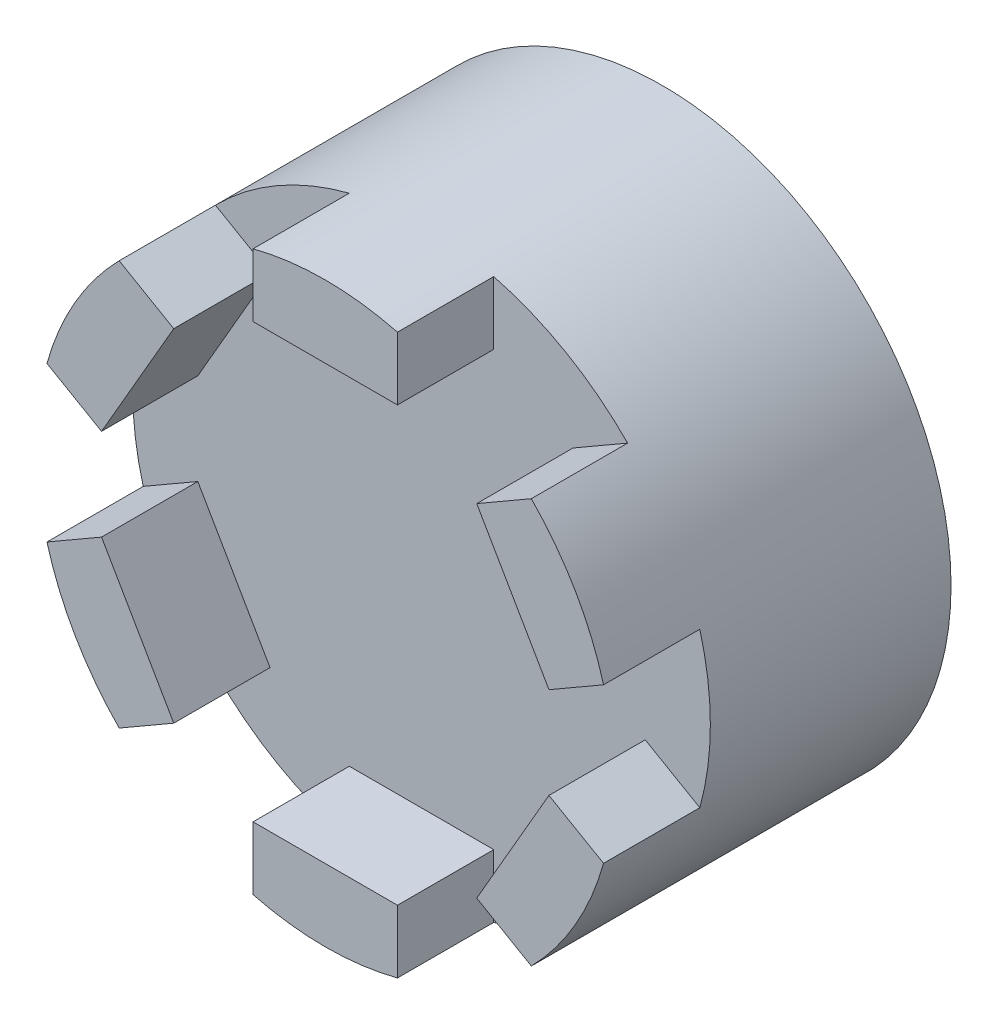
SolidWorks part; units mm, degrees
ref_plane "前视基准面" through (0, 0, 0) normal (0, 0, 1) x (1, 0, 0)
ref_plane "上视基准面" through (0, 0, 0) normal (0, 1, 0) x (1, 0, 0)
ref_plane "右视基准面" through (0, 0, 0) normal (1, 0, 0) x (0, 0, -1)
other "Configuration Table"
sketch "草图1" plane through (0, 0, 0) normal (0, 0, 1) x (1, 0, 0)
  circle A0 centre (0, 0) radius 15
  dimension "D1" = 30
sketch "草图2" plane through (0, 0, 0) normal (0, 0, 1) x (1, 0, 0)
  circle A0 centre (0, 0) radius 60
  dimension "D1" = 120
extrude "凸台-拉伸1" add sketch "草图2" along normal blind 50 contours A0
extrude "切除-拉伸1" cut sketch "草图1" along normal blind 30 contours A0
sketch "草图3" plane through (0, 0, 50) normal (0, 0, 1) x (1, 0, 0)
  line L0 (42.8115, 42.0378) -> (31.4711, 35.4904)
  line L2 (-15, 58.0948) -> (-15, 45)
  line L3 (-15, 45) -> (15, 45)
  line L4 (15, 58.0948) -> (15, 45)
  line L5 (57.8115, 16.057) -> (46.4711, 9.5096)
  line L6 (31.4711, 35.4904) -> (46.4711, 9.5096)
  line L7 (57.8115, -16.057) -> (46.4711, -9.5096)
  line L8 (42.8115, -42.0378) -> (31.4711, -35.4904)
  line L9 (46.4711, -9.5096) -> (31.4711, -35.4904)
  line L10 (15, -58.0948) -> (15, -45)
  line L11 (-15, -58.0948) -> (-15, -45)
  line L12 (15, -45) -> (-15, -45)
  line L13 (-42.8115, -42.0378) -> (-31.4711, -35.4904)
  line L14 (-57.8115, -16.057) -> (-46.4711, -9.5096)
  line L15 (-31.4711, -35.4904) -> (-46.4711, -9.5096)
  line L16 (-57.8115, 16.057) -> (-46.4711, 9.5096)
  line L17 (-42.8115, 42.0378) -> (-31.4711, 35.4904)
  line L18 (-46.4711, 9.5096) -> (-31.4711, 35.4904)
  arc A0 (57.8115, 16.057) -> (42.8115, 42.0378) centre (0, 0) ccw
  circle A1 centre (0, 0) radius 60
  arc A2 (15, 58.0948) -> (-15, 58.0948) centre (0, 0) ccw
  arc A3 (42.8115, -42.0378) -> (57.8115, -16.057) centre (0, 0) ccw
  arc A4 (-15, -58.0948) -> (15, -58.0948) centre (0, 0) ccw
  arc A5 (-57.8115, -16.057) -> (-42.8115, -42.0378) centre (0, 0) ccw
  arc A6 (-42.8115, 42.0378) -> (-57.8115, 16.057) centre (0, 0) ccw
  point P7 (0, 45)
  dimension "D2" = 30
  dimension "D3" = 45
  dimension "D1" = 0
  dimension "D4" = 6
extrude "凸台-拉伸2" add sketch "草图3" along normal blind 20
sketch "草图5" plane through (0, 0, 0) normal (0, 0, -1) x (-1, 0, 0)
  line L1 (-5, 17) -> (5, 17)
  line L2 (-5, 17) -> (-5, 10.1153)
  line L3 (-5, 10.1153) -> (5, 10.1153)
  line L4 (5, 17) -> (5, 10.1153)
  point P4 (0, 10.1153)
  dimension "D1" = 10
  dimension "D2" = 17
extrude "切除-拉伸2" cut sketch "草图5" against normal blind 15 contours L4 L3 L2 L1
